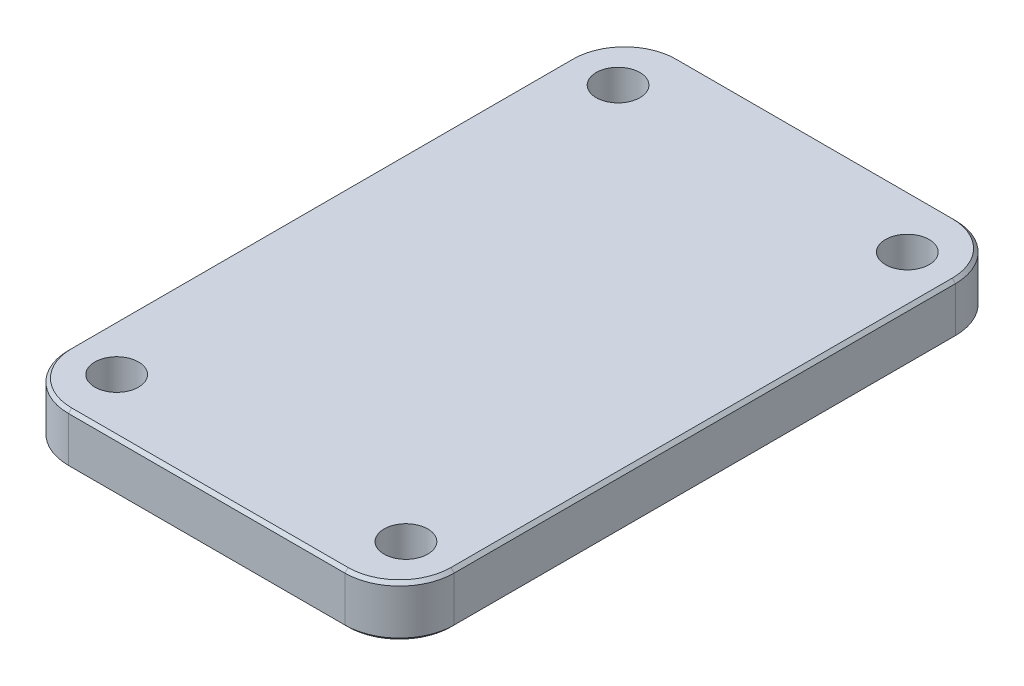
SolidWorks part; units mm, degrees
ref_plane "Front Plane" through (0, 0, 0) normal (0, 0, 1) x (1, 0, 0)
ref_plane "Top Plane" through (0, 0, 0) normal (0, 1, 0) x (1, 0, 0)
ref_plane "Right Plane" through (0, 0, 0) normal (1, 0, 0) x (0, 0, -1)
ref_plane "Plane4" through (0, -8, 0) normal (0, -1, 0) x (1, 0, 0)
sketch "Sketch1" plane through (0, -8, 0) normal (0, -1, 0) x (1, 0, 0)
  line L0 (-30, -50) -> (30, -50)
  line L1 (30, -50) -> (30, 45)
  line L2 (30, 45) -> (-30, 45)
  line L3 (-30, 45) -> (-30, -50)
  dimension "D1" = 60
  dimension "D2" = 95
  dimension "D3" = 45
  dimension "D4" = 30
extrude "Boss-Extrude1" add sketch "Sketch1" against normal blind 8
hole_wizard "Ø6.8 (6.8) Diameter Hole1" positions "Sketch3" profile "Sketch2" hole size "Ø6.8" standard "ANSI Metric"
sketch "Sketch3" plane through (0, -8, 0) normal (0, -1, 0) x (-1, 0, 0)
  line L0 (-30, 50) -> (-30, -45) construction
  line L1 (30, -45) -> (30, 50) construction
  line L2 (30, 50) -> (-30, 50) construction
  line L3 (-30, -45) -> (30, -45) construction
  point P0 (22.5, 41.5)
  point P1 (-22.5, 41.5)
  point P2 (-22.5, -36.5)
  point P3 (22.5, -36.5)
  dimension "D1" = 7.5
  dimension "D2" = 7.5
  dimension "D3" = 8.5
  dimension "D4" = 8.5
  dimension "D5" = 8.5
  dimension "D6" = 8.5
  dimension "D7" = 7.5
  dimension "D8" = 7.5
sketch "Sketch2" plane through (-22.5, -8, -41.5) normal (1, 0, 0) x (0, 0, -1)
  line L0 (0, 0) -> (0, 8)
  line L1 (0, 8) -> (3.4, 8)
  line L2 (3.4, 8) -> (3.4, 0)
  line L5 (3.4, 0) -> (0, 0)
  line L11 (0, -6.35) -> (0, 107.95) construction
  dimension "通孔孔直径" = 6.8
  dimension "通孔孔深度" = 8
fillet "Fillet1" radius 8.5 4 edges at (30, -4, -50) (30, -4, 45) (-30, -4, -50) (-30, -4, 45)
chamfer "Chamfer1" distance 0.5 angle 45 16 edges at (30, 0, -2.5) (27.5104, 0, 42.5104) (27.5104, 0, -47.5104) (0, 0, 45) (0, 0, -50) (-27.5104, 0, 42.5104) (-27.5104, 0, -47.5104) (-30, 0, -2.5) (-27.5104, -8, 42.5104) (0, -8, 45) (-30, -8, -2.5) (27.5104, -8, 42.5104) (-27.5104, -8, -47.5104) (30, -8, -2.5) (0, -8, -50) (27.5104, -8, -47.5104)
